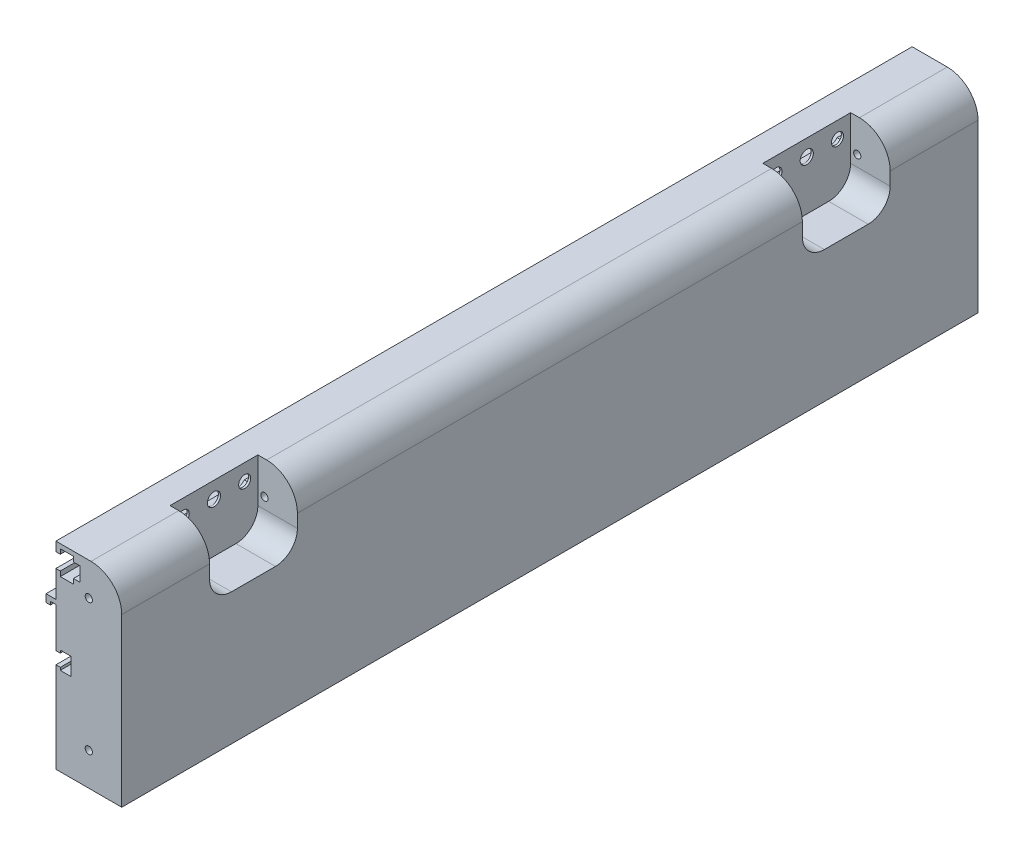
from build123d import *

# Parameters (mm, degrees)
SKETCH1_R                                  = 1.65
BOSS_EXTRUDE1_DEPTH                        = 195
SKETCH2_R                                  = 11
CUT_EXTRUDE1_DEPTH                         = 7
SKETCH3_R                                  = 3
CUT_EXTRUDE2_DEPTH                         = 217.852484422
CUT_EXTRUDE4_DEPTH                         = 18
M5_SOCKET_HEAD_CAP_SCREW_TYPE1_D           = 5.5
M5_SOCKET_HEAD_CAP_SCREW_TYPE1_CBORE_D     = 10
M5_SOCKET_HEAD_CAP_SCREW_TYPE1_CBORE_DEPTH = 11


with BuildPart() as part:
    # Sketch1 → Boss-Extrude1 (new, symmetric)
    with BuildSketch(Plane.XY):
        with BuildLine():
            Line((0, 0), (0, 41.2))
            Line((0, 41.2), (2, 41.2))
            Line((2, 41.2), (2, 40))
            Line((2, 40), (7, 40))
            Line((7, 40), (7, 48))
            Line((7, 48), (2, 48))
            Line((2, 48), (2, 46.8))
            Line((2, 46.8), (0, 46.8))
            Line((0, 46.8), (0, 65))
            Line((0, 65), (-2.5, 65))
            Line((-2.5, 65), (-2.5, 63.5))
            Line((-2.5, 63.5), (-4.5, 63.5))
            Line((-4.5, 63.5), (-4.5, 67))
            Line((-4.5, 67), (0, 67))
            Line((0, 67), (0, 79.2))
            Line((0, 79.2), (2, 79.2))
            Line((2, 79.2), (2, 77))
            Line((2, 77), (8, 77))
            Line((8, 77), (8, 79.25))
            Line((8, 79.25), (11, 79.25))
            Line((11, 79.25), (11, 85.75))
            Line((11, 85.75), (8, 85.75))
            Line((8, 85.75), (8, 88))
            Line((8, 88), (2, 88))
            Line((2, 88), (2, 85.8))
            Line((2, 85.8), (0, 85.8))
            Line((0, 85.8), (0, 90))
            Line((0, 90), (16, 90))
            ThreePointArc((16, 90), (25.899494937, 85.899494937), (30, 76))
            Line((30, 76), (30, 0))
            Line((30, 0), (0, 0))
        make_face()
        with Locations((15, 75)):
            Circle(SKETCH1_R, mode=Mode.SUBTRACT)
        with Locations(Location((15, 15, 0), (0, 0, 180))):
            Circle(SKETCH1_R, mode=Mode.SUBTRACT)
    extrude(amount=BOSS_EXTRUDE1_DEPTH, both=True)

    # Sketch2 → Cut-Extrude1 (cut)
    with BuildSketch(Plane.ZY):
        with Locations((-155, 44)):
            Circle(SKETCH2_R)
        with Locations((155, 44)):
            Circle(SKETCH2_R)
    extrude(amount=-CUT_EXTRUDE1_DEPTH, mode=Mode.SUBTRACT)

    # Sketch3 → Cut-Extrude2 (cut, through all)
    with BuildSketch(Plane.ZY):
        with Locations(Location((-135, 82.5, 0), (0, 0, 270))):
            Circle(SKETCH3_R)
        with Locations(Location((135, 82.5, 0), (0, 0, 270))):
            Circle(SKETCH3_R)
    cut_extrude2 = extrude(amount=-CUT_EXTRUDE2_DEPTH, mode=Mode.SUBTRACT)

    # Sketch9 → Cut-Extrude4 (cut)
    with BuildSketch(Plane(origin=(30, 0, 0), x_dir=(0, 0, -1), z_dir=(1, 0, 0))):
        with BuildLine():
            Line((-155, 90), (-115, 90))
            Line((-115, 90), (-115, 70))
            ThreePointArc((-115, 70), (-117.928932188, 62.928932188), (-125, 60))
            Line((-125, 60), (-145, 60))
            ThreePointArc((-145, 60), (-152.071067812, 62.928932188), (-155, 70))
            Line((-155, 70), (-155, 90))
        make_face()
    cut_extrude4 = extrude(amount=-CUT_EXTRUDE4_DEPTH, mode=Mode.SUBTRACT)

    # M5 socket head cap screw type1 (through all)
    with Locations(Plane.ZY):
        with Locations((149, 82.5), (121, 82.5)):
            m5_socket_head_cap_screw_type1 = CounterBoreHole(M5_SOCKET_HEAD_CAP_SCREW_TYPE1_D / 2, M5_SOCKET_HEAD_CAP_SCREW_TYPE1_CBORE_D / 2, M5_SOCKET_HEAD_CAP_SCREW_TYPE1_CBORE_DEPTH)

    # Mirror2: Cut-Extrude2, Cut-Extrude4, M5 socket head cap screw type1 across plane
    add(cut_extrude2.mirror(Plane.XY), mode=Mode.SUBTRACT)
    add(cut_extrude4.mirror(Plane.XY), mode=Mode.SUBTRACT)
    add(m5_socket_head_cap_screw_type1.mirror(Plane.XY), mode=Mode.SUBTRACT)


solid = part.part
